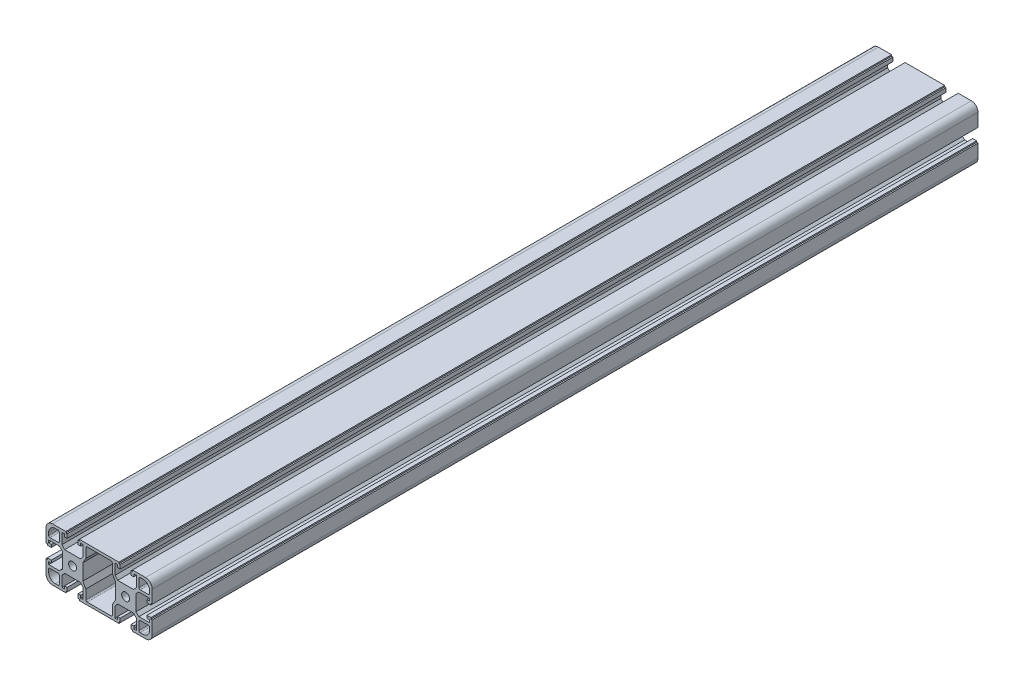
from build123d import *

# Parameters (mm, degrees)
SKETCH_1_R          = 3
SKETCH_1_W          = 8
SKETCH_1_H          = 8
EXTRUDE_1_DEPTH     = 323.5
FILLET_1_R          = 5
FILLET_2_R          = 1
CUT_EXTRUDE_1_DEPTH = 25


with BuildPart() as part:
    # 草图1 → 拉伸1 (new, symmetric)
    with BuildSketch(Plane.XY):
        Polygon((-5.1, 20), (-5.1, 19), (-4.1, 19), (-4.1, 16), (-6.1, 16), (-6.1, 18), (-8, 18), (-8, 10), (-6, 7.7), (6, 7.7), (8, 10), (8, 18), (6.1, 18), (6.1, 16), (4.1, 16), (4.1, 19), (5.1, 19), (5.1, 20), (34.9, 20), (34.9, 19), (35.9, 19), (35.9, 16), (33.9, 16), (33.9, 18), (32, 18), (32, 10), (34, 7.7), (46, 7.7), (48, 10), (48, 18), (46.1, 18), (46.1, 16), (44.1, 16), (44.1, 19), (45.1, 19), (45.1, 20), (60, 20), (60, 5.1), (59, 5.1), (59, 4.1), (56, 4.1), (56, 6.1), (58, 6.1), (58, 8), (50, 8), (47.7, 6), (47.7, -6), (50, -8), (58, -8), (58, -6.1), (56, -6.1), (56, -4.1), (59, -4.1), (59, -5.1), (60, -5.1), (60, -20), (45.1, -20), (45.1, -19), (44.1, -19), (44.1, -16), (46.1, -16), (46.1, -18), (48, -18), (48, -10), (46, -7.7), (34, -7.7), (32, -10), (32, -18), (33.9, -18), (33.9, -16), (35.9, -16), (35.9, -19), (34.9, -19), (34.9, -20), (5.1, -20), (5.1, -19), (4.1, -19), (4.1, -16), (6.1, -16), (6.1, -18), (8, -18), (8, -10), (6, -7.7), (-6, -7.7), (-8, -10), (-8, -18), (-6.1, -18), (-6.1, -16), (-4.1, -16), (-4.1, -19), (-5.1, -19), (-5.1, -20), (-20, -20), (-20, -5.1), (-19, -5.1), (-19, -4.1), (-16, -4.1), (-16, -6.1), (-18, -6.1), (-18, -8), (-10, -8), (-7.7, -6), (-7.7, 6), (-10, 8), (-18, 8), (-18, 6.1), (-16, 6.1), (-16, 4.1), (-19, 4.1), (-19, 5.1), (-20, 5.1), (-20, 20), align=None)
        with Locations(Location((0, 0, 0), (0, 0, 180))):
            Circle(SKETCH_1_R, mode=Mode.SUBTRACT)
        with Locations(Location((40, 0, 0), (0, 0, 180))):
            Circle(SKETCH_1_R, mode=Mode.SUBTRACT)
        Polygon((7.7, 6), (10, 10), (10, 18), (30, 18), (30, 10), (32.3, 6), (32.3, -6), (30, -10), (30, -18), (10, -18), (10, -10), (7.7, -6), align=None, mode=Mode.SUBTRACT)
        with Locations((-14, 14)):
            Rectangle(SKETCH_1_W, SKETCH_1_H, mode=Mode.SUBTRACT)
        with Locations((-14, -14)):
            Rectangle(SKETCH_1_W, SKETCH_1_H, mode=Mode.SUBTRACT)
        with Locations((54, -14)):
            Rectangle(SKETCH_1_W, SKETCH_1_H, mode=Mode.SUBTRACT)
        with Locations((54, 14)):
            Rectangle(SKETCH_1_W, SKETCH_1_H, mode=Mode.SUBTRACT)
    extrude(amount=EXTRUDE_1_DEPTH, both=True)

    # 圆角1
    fillet_1_edges = [part.edges().sort_by_distance(p)[0] for p in [
        (-20, 20, 0),
        (60, 20, 0),
        (60, -20, 0),
        (-20, -20, 0),
        (-18, 18, 0),
        (-18, -18, 0),
        (58, -18, 0),
        (58, 18, 0),
    ]]
    fillet(fillet_1_edges, radius=FILLET_1_R)

    # 圆角2
    fillet_2_edges = [part.edges().sort_by_distance(p)[0] for p in [
        (10, -18, 0),
        (30, -18, 0),
        (30, 18, 0),
        (10, 18, 0),
        (-18, 10, 0),
        (-10, 10, 0),
        (-10, 18, 0),
        (-10, -18, 0),
        (-10, -10, 0),
        (-18, -10, 0),
        (58, -10, 0),
        (50, -10, 0),
        (50, -18, 0),
        (50, 18, 0),
        (50, 10, 0),
        (58, 10, 0),
    ]]
    fillet(fillet_2_edges, radius=FILLET_2_R)

    # 草图4 → 切除-拉伸1 (cut)
    with BuildSketch(Plane(origin=(0, 0, -323.5), x_dir=(-1, 0, 0), z_dir=(0, 0, -1))):
        with BuildLine():
            Line((-60, -5.1), (-60, -15))
            ThreePointArc((-60, -15), (-58.535533906, -18.535533906), (-55, -20))
            Line((-55, -20), (-45.1, -20))
            Line((-45.1, -20), (-45.1, -19))
            Line((-45.1, -19), (-44.1, -19))
            Line((-44.1, -19), (-44.1, -16))
            Line((-44.1, -16), (-46.1, -16))
            Line((-46.1, -16), (-46.1, -18))
            Line((-46.1, -18), (-48, -18))
            Line((-48, -18), (-48, -10))
            Line((-48, -10), (-46, -7.7))
            Line((-46, -7.7), (-34, -7.7))
            Line((-34, -7.7), (-32, -10))
            Line((-32, -10), (-32, -18))
            Line((-32, -18), (-33.9, -18))
            Line((-33.9, -18), (-33.9, -16))
            Line((-33.9, -16), (-35.9, -16))
            Line((-35.9, -16), (-35.9, -19))
            Line((-35.9, -19), (-34.9, -19))
            Line((-34.9, -19), (-34.9, -20))
            Line((-34.9, -20), (-5.1, -20))
            Line((-5.1, -20), (-5.1, -19))
            Line((-5.1, -19), (-4.1, -19))
            Line((-4.1, -19), (-4.1, -16))
            Line((-4.1, -16), (-6.1, -16))
            Line((-6.1, -16), (-6.1, -18))
            Line((-6.1, -18), (-8, -18))
            Line((-8, -18), (-8, -10))
            Line((-8, -10), (-6, -7.7))
            Line((-6, -7.7), (6, -7.7))
            Line((6, -7.7), (8, -10))
            Line((8, -10), (8, -18))
            Line((8, -18), (6.1, -18))
            Line((6.1, -18), (6.1, -16))
            Line((6.1, -16), (4.1, -16))
            Line((4.1, -16), (4.1, -19))
            Line((4.1, -19), (5.1, -19))
            Line((5.1, -19), (5.1, -20))
            Line((5.1, -20), (15, -20))
            ThreePointArc((15, -20), (18.535533906, -18.535533906), (20, -15))
            Line((20, -15), (20, -5.1))
            Line((20, -5.1), (19, -5.1))
            Line((19, -5.1), (19, -4.1))
            Line((19, -4.1), (16, -4.1))
            Line((16, -4.1), (16, -6.1))
            Line((16, -6.1), (18, -6.1))
            Line((18, -6.1), (18, -8))
            Line((18, -8), (10, -8))
            Line((10, -8), (7.7, -6))
            Line((7.7, -6), (7.7, 6))
            Line((7.7, 6), (10, 8))
            Line((10, 8), (18, 8))
            Line((18, 8), (18, 6.1))
            Line((18, 6.1), (16, 6.1))
            Line((16, 6.1), (16, 4.1))
            Line((16, 4.1), (19, 4.1))
            Line((19, 4.1), (19, 5.1))
            Line((19, 5.1), (20, 5.1))
            Line((20, 5.1), (20, 15))
            ThreePointArc((20, 15), (18.535533906, 18.535533906), (15, 20))
            Line((15, 20), (5.1, 20))
            Line((5.1, 20), (5.1, 19))
            Line((5.1, 19), (4.1, 19))
            Line((4.1, 19), (4.1, 16))
            Line((4.1, 16), (6.1, 16))
            Line((6.1, 16), (6.1, 18))
            Line((6.1, 18), (8, 18))
            Line((8, 18), (8, 10))
            Line((8, 10), (6, 7.7))
            Line((6, 7.7), (-6, 7.7))
            Line((-6, 7.7), (-8, 10))
            Line((-8, 10), (-8, 18))
            Line((-8, 18), (-6.1, 18))
            Line((-6.1, 18), (-6.1, 16))
            Line((-6.1, 16), (-4.1, 16))
            Line((-4.1, 16), (-4.1, 19))
            Line((-4.1, 19), (-5.1, 19))
            Line((-5.1, 19), (-5.1, 20))
            Line((-5.1, 20), (-34.9, 20))
            Line((-34.9, 20), (-34.9, 19))
            Line((-34.9, 19), (-35.9, 19))
            Line((-35.9, 19), (-35.9, 16))
            Line((-35.9, 16), (-33.9, 16))
            Line((-33.9, 16), (-33.9, 18))
            Line((-33.9, 18), (-32, 18))
            Line((-32, 18), (-32, 10))
            Line((-32, 10), (-34, 7.7))
            Line((-34, 7.7), (-46, 7.7))
            Line((-46, 7.7), (-48, 10))
            Line((-48, 10), (-48, 18))
            Line((-48, 18), (-46.1, 18))
            Line((-46.1, 18), (-46.1, 16))
            Line((-46.1, 16), (-44.1, 16))
            Line((-44.1, 16), (-44.1, 19))
            Line((-44.1, 19), (-45.1, 19))
            Line((-45.1, 19), (-45.1, 20))
            Line((-45.1, 20), (-55, 20))
            ThreePointArc((-55, 20), (-58.535533906, 18.535533906), (-60, 15))
            Line((-60, 15), (-60, 5.1))
            Line((-60, 5.1), (-59, 5.1))
            Line((-59, 5.1), (-59, 4.1))
            Line((-59, 4.1), (-56, 4.1))
            Line((-56, 4.1), (-56, 6.1))
            Line((-56, 6.1), (-58, 6.1))
            Line((-58, 6.1), (-58, 8))
            Line((-58, 8), (-50, 8))
            Line((-50, 8), (-47.7, 6))
            Line((-47.7, 6), (-47.7, -6))
            Line((-47.7, -6), (-50, -8))
            Line((-50, -8), (-58, -8))
            Line((-58, -8), (-58, -6.1))
            Line((-58, -6.1), (-56, -6.1))
            Line((-56, -6.1), (-56, -4.1))
            Line((-56, -4.1), (-59, -4.1))
            Line((-59, -4.1), (-59, -5.1))
            Line((-59, -5.1), (-60, -5.1))
        make_face()
    extrude(amount=-CUT_EXTRUDE_1_DEPTH, mode=Mode.SUBTRACT)


solid = part.part
